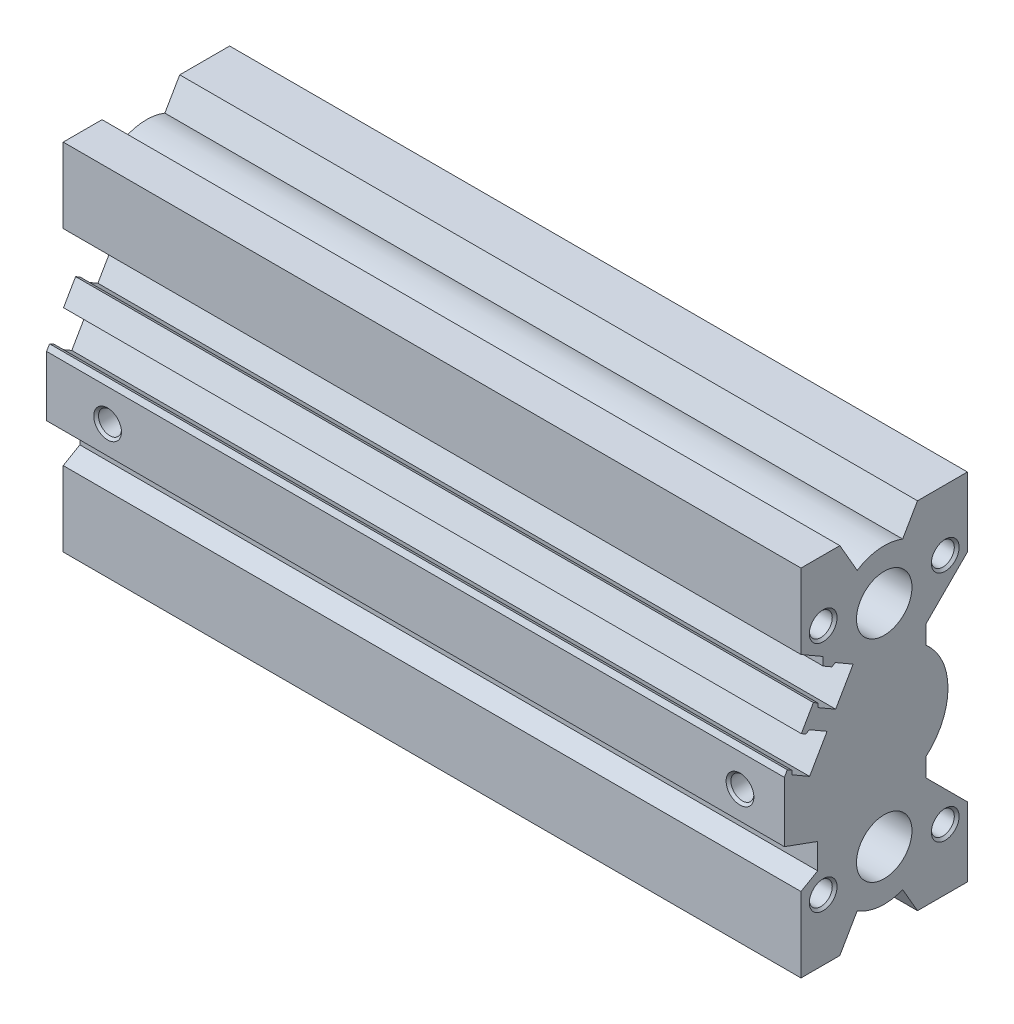
from build123d import *

# Parameters (mm, degrees)
SKETCH_1_W                  = 33
SKETCH_1_H                  = 64
EXTRUDE_1_DEPTH             = 133
HOLE_WIZARD_1_D             = 10
PATTERN_LINEAR_1_COUNT      = 2
PATTERN_LINEAR_1_PITCH      = 38
PATTERN_LINEAR_2_COUNT      = 2
PATTERN_LINEAR_2_PITCH      = 22
PATTERN_LINEAR_2_COUNT_DIR2 = 2
PATTERN_LINEAR_2_PITCH_DIR2 = 42
PATTERN_LINEAR_3_COUNT      = 2
PATTERN_LINEAR_3_PITCH      = 107
PATTERN_LINEAR_3_COUNT_DIR2 = 2
PATTERN_LINEAR_3_PITCH_DIR2 = 54
CUT_EXTRUDE_1_DEPTH         = 133
CUT_EXTRUDE_2_DEPTH         = 133
CUT_EXTRUDE_3_DEPTH         = 133
CUT_EXTRUDE_4_DEPTH         = 133
CUT_EXTRUDE_5_DEPTH         = 133
HOLE_WIZARD_4_D             = 4.134
HOLE_WIZARD_4_DEPTH         = 6
HOLE_WIZARD_4_CSINK_D       = 5
HOLE_WIZARD_4_CSINK_ANGLE   = 90
PATTERN_LINEAR_4_COUNT      = 2
PATTERN_LINEAR_4_PITCH      = 114


with BuildPart() as part:
    # 草图1 → 凸台-拉伸1 (new body)
    with BuildSketch(Plane(origin=(0, 0, 0), x_dir=(0, 0, -1), z_dir=(1, 0, 0))):
        with Locations((-1.5, 0)):
            Rectangle(SKETCH_1_W, SKETCH_1_H)
    extrude(amount=EXTRUDE_1_DEPTH)

    # 孔1 (through all)
    with Locations(Plane(origin=(133, 0, 0), x_dir=(0, 0, -1), z_dir=(1, 0, 0))):
        with Locations((0, 19)):
            hole_wizard_1 = Hole(HOLE_WIZARD_1_D / 2)

    # 阵列(线性)1: 孔1 ×2
    with Locations(*[(0, -i * PATTERN_LINEAR_1_PITCH, 0) for i in range(1, PATTERN_LINEAR_1_COUNT)]):
        add(hole_wizard_1, mode=Mode.SUBTRACT)

    # 草图5 → 孔2 (revolve, cut)
    with BuildSketch(Plane(origin=(133, 21, 11), x_dir=(0, 0, -1), z_dir=(0, 1, 0))):
        Polygon((0, 0), (0, 14.099043395), (2.067, 13), (2.067, 0.433), (2.5, 0), align=None)
    hole_wizard_2 = revolve(axis=Axis((147.308894879, 21, 11), (-1, 0, 0)), mode=Mode.SUBTRACT)

    # 阵列(线性)2: Hole Wizard 2 2 × 2
    with Locations(*[(0, -j * PATTERN_LINEAR_2_PITCH_DIR2, -i * PATTERN_LINEAR_2_PITCH) for i in range(PATTERN_LINEAR_2_COUNT) for j in range(PATTERN_LINEAR_2_COUNT_DIR2) if (i, j) != (0, 0)]):
        add(hole_wizard_2, mode=Mode.SUBTRACT)

    # 草图8 → 孔3 (revolve, cut)
    with BuildSketch(Plane(origin=(13, 27, -15), x_dir=(0, 1, 0), z_dir=(1, 0, 0))):
        Polygon((0, 0), (0, 9.099043395), (2.067, 8), (2.067, 0.433), (2.5, 0), align=None)
    hole_wizard_3 = revolve(axis=Axis((13, 27, -29.308894879), (0, 0, 1)), mode=Mode.SUBTRACT)

    # 阵列(线性)3: Hole Wizard 3 2 × 2
    with Locations(*[(i * PATTERN_LINEAR_3_PITCH, -j * PATTERN_LINEAR_3_PITCH_DIR2, 0) for i in range(PATTERN_LINEAR_3_COUNT) for j in range(PATTERN_LINEAR_3_COUNT_DIR2) if (i, j) != (0, 0)]):
        add(hole_wizard_3, mode=Mode.SUBTRACT)

    # 草图11 → 切除-旋转1 (revolve, cut)
    with BuildSketch(Plane.XY, mode=Mode.PRIVATE) as cut_revolve_1_sk:
        Polygon((0, 0), (0, 4), (16.5, 4), (16.5, 8), (121.5, 8), (121.5, 0), align=None)
    revolve(cut_revolve_1_sk.sketch.rotate(Axis((121.5, 0, 0), (-1, 0, 0)), 270), axis=Axis((121.5, 0, 0), (-1, 0, 0)), mode=Mode.SUBTRACT)

    # 草图12 → 切除-拉伸1 (cut)
    with BuildSketch(Plane(origin=(0, 0, 0), x_dir=(0, 0, -1), z_dir=(1, 0, 0))):
        with BuildLine():
            Line((-8, 32), (-4.865738712, 26.571300205))
            ThreePointArc((-4.865738712, 26.571300205), (-0.867061595, 27.958136201), (3.323361728, 27.36392652))
            Line((3.323361728, 27.36392652), (6, 32))
            Line((6, 32), (-8, 32))
        make_face()
    extrude(amount=CUT_EXTRUDE_1_DEPTH, mode=Mode.SUBTRACT)

    # 草图13 → 切除-拉伸2 (cut)
    with BuildSketch(Plane(origin=(0, 0, 0), x_dir=(0, 0, -1), z_dir=(1, 0, 0))):
        with BuildLine():
            Line((-8, -32), (6, -32))
            Line((6, -32), (3.323361728, -27.36392652))
            ThreePointArc((3.323361728, -27.36392652), (-0.867061595, -27.958136201), (-4.865738712, -26.571300205))
            Line((-4.865738712, -26.571300205), (-8, -32))
        make_face()
    extrude(amount=CUT_EXTRUDE_2_DEPTH, mode=Mode.SUBTRACT)

    # 草图14 → 切除-拉伸3 (cut)
    with BuildSketch(Plane(origin=(0, 0, 0), x_dir=(0, 0, -1), z_dir=(1, 0, 0))):
        with BuildLine():
            Line((7.5, -12), (15, -19.5))
            Line((15, -19.5), (15, 19.5))
            Line((15, 19.5), (7.5, 12))
            Line((7.5, 12), (7.5, 8.717797887))
            ThreePointArc((7.5, 8.717797887), (11.5, 0), (7.5, -8.717797887))
            Line((7.5, -8.717797887), (7.5, -12))
        make_face()
    extrude(amount=CUT_EXTRUDE_3_DEPTH, mode=Mode.SUBTRACT)

    # 草图15 → 切除-拉伸4 (cut)
    with BuildSketch(Plane(origin=(0, 0, 0), x_dir=(0, 0, -1), z_dir=(1, 0, 0))):
        Polygon((-18, -32), (-15, -32), (-15, -18.5), (-12, -16.767949192), (-12, -12.183821406), (-18, -10), align=None)
    extrude(amount=CUT_EXTRUDE_4_DEPTH, mode=Mode.SUBTRACT)

    # 草图16 → 切除-拉伸5 (cut)
    with BuildSketch(Plane(origin=(0, 0, 0), x_dir=(0, 0, -1), z_dir=(1, 0, 0))):
        Polygon((-18, 32), (-18, 0.8235), (-17.4691, 1.743045774), (-16.655766975, 1.273467733), (-16.655766975, 0.551779896), (-13.451472981, -1.298220104), (-10.301472981, 4.15773994), (-13.505766975, 6.00773994), (-14.130766975, 5.646896022), (-14.9441, 6.116474063), (-12.76915, 9.883597967), (-11.955816975, 9.414019926), (-11.955816975, 8.692332089), (-8.751522981, 6.842332089), (-5.601522981, 12.298292133), (-8.805816975, 14.148292133), (-9.430816975, 13.787448215), (-11, 14.693416457), (-11, 16.190598923), (-15, 18.5), (-15, 32), align=None)
    extrude(amount=CUT_EXTRUDE_5_DEPTH, mode=Mode.SUBTRACT)

    # 孔4
    with Locations(Plane.XY.offset(18)):
        with Locations((11, -5)):
            hole_wizard_4 = CounterSinkHole(HOLE_WIZARD_4_D / 2, HOLE_WIZARD_4_CSINK_D / 2, depth=HOLE_WIZARD_4_DEPTH, counter_sink_angle=HOLE_WIZARD_4_CSINK_ANGLE)

    # 阵列(线性)4: 孔4 ×2
    with Locations(*[(i * PATTERN_LINEAR_4_PITCH, 0, 0) for i in range(1, PATTERN_LINEAR_4_COUNT)]):
        add(hole_wizard_4, mode=Mode.SUBTRACT)


solid = part.part
